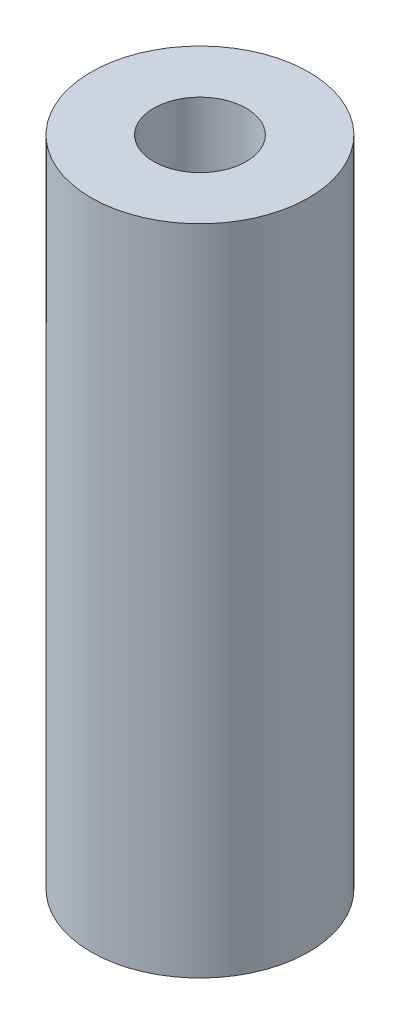
from build123d import *

# Parameters (mm, degrees)
SKETCH1_R             = 8
BOSS_EXTRUDE1_DEPTH   = 48
M8_TAPPED_HOLE1_D     = 6.8
M8_TAPPED_HOLE1_DEPTH = 26
M8_TAPPED_HOLE1_TIP   = 2.042926105


with BuildPart() as part:
    # Sketch1 → Boss-Extrude1 (new body)
    with BuildSketch(Plane(origin=(0, 0, 0), x_dir=(1, 0, 0), z_dir=(0, 1, 0))):
        with Locations(Location((0, 0, 0), (0, 0, 270))):
            Circle(SKETCH1_R)
    extrude(amount=BOSS_EXTRUDE1_DEPTH)

    # M8 Tapped Hole1
    with Locations(Plane(origin=(0, 48, 0), x_dir=(1, 0, 0), z_dir=(0, 1, 0))):
        with Locations((0, 0)):
            Hole(M8_TAPPED_HOLE1_D / 2, depth=M8_TAPPED_HOLE1_DEPTH)
            with Locations((0, 0, -(M8_TAPPED_HOLE1_DEPTH + M8_TAPPED_HOLE1_TIP / 2))):  # 118° drill point
                Cone(0, M8_TAPPED_HOLE1_D / 2, M8_TAPPED_HOLE1_TIP, mode=Mode.SUBTRACT)


solid = part.part
